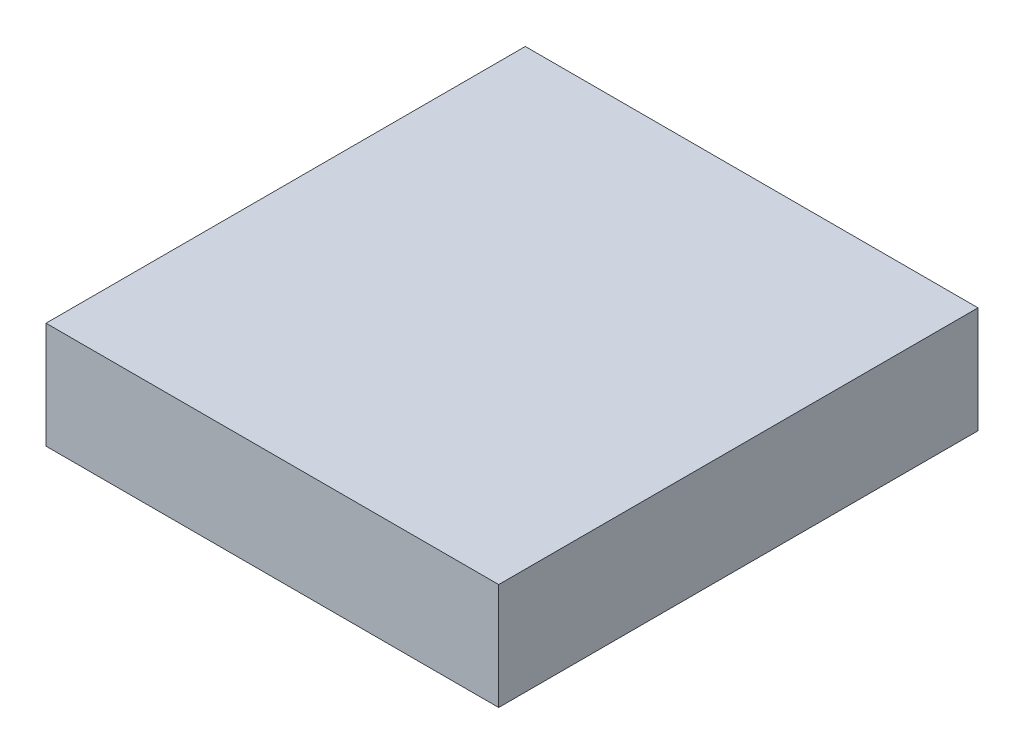
SolidWorks part; units mm, degrees
material "标准件"
ref_plane "前视基准面" through (0, 0, 0) normal (0, 0, 1) x (1, 0, 0)
ref_plane "上视基准面" through (0, 0, 0) normal (0, 1, 0) x (1, 0, 0)
ref_plane "右视基准面" through (0, 0, 0) normal (1, 0, 0) x (0, 0, -1)
sketch "草图1" plane through (0, 0, 0) normal (0, 1, 0) x (1, 0, 0)
  line L1 (-85, -90) -> (85, -90)
  line L2 (-85, -90) -> (-85, 90)
  line L3 (-85, 90) -> (85, 90)
  line L4 (85, -90) -> (85, 90)
  line L5 (-85, -90) -> (85, 90) construction
  line L6 (-85, 90) -> (85, -90) construction
  point P0 (0, 0)
  dimension "D1" = 170
  dimension "D2" = 180
extrude "凸台-拉伸1" add sketch "草图1" along normal blind 40
